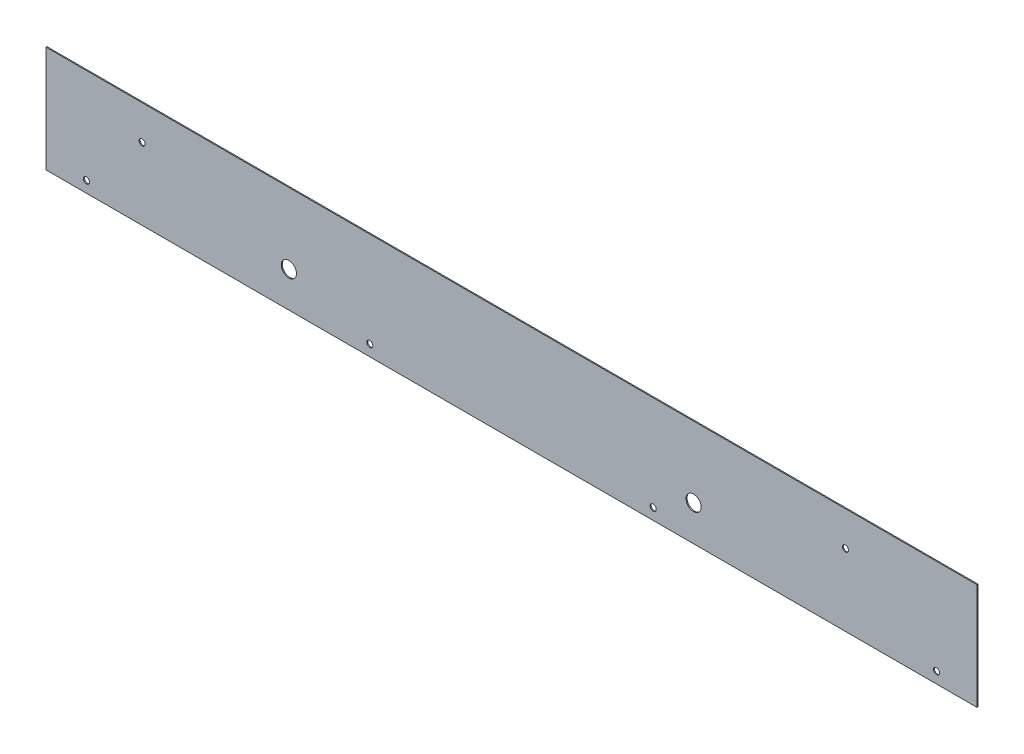
from build123d import *

# Parameters (mm, degrees)
SKETCH1_W                = 920
SKETCH1_H                = 1
EXTRUDE1_DEPTH           = 52.5
SKETCH2_R                = 7.5
CUT_EXTRUDE1_DEPTH       = 463.987310841
M5_CLEARANCE_HOLE1_D     = 6
M5_CLEARANCE_HOLE1_DEPTH = 7
M5_CLEARANCE_HOLE1_TIP   = 1.802581857


with BuildPart() as part:
    # Sketch1 → Extrude1 (new, symmetric)
    with BuildSketch(Plane(origin=(0, 0, 0), x_dir=(1, 0, 0), z_dir=(0, 1, 0))):
        Rectangle(SKETCH1_W, SKETCH1_H)
    extrude(amount=EXTRUDE1_DEPTH, both=True)

    # Sketch2 → Cut-Extrude1 (cut, through all)
    with BuildSketch(Plane.XY.offset(0.5)):
        with Locations((-220, -17.5)):
            Circle(SKETCH2_R)
        with Locations((180, -17.5)):
            Circle(SKETCH2_R)
    extrude(amount=-CUT_EXTRUDE1_DEPTH, mode=Mode.SUBTRACT)

    # M5 Clearance Hole1
    with Locations(Plane.XY.offset(0.5)):
        with Locations((-420, -41.5), (-140, -41.5), (140, -41.5), (-365, 18.5), (330, 18.5), (420, -41.5)):
            Hole(M5_CLEARANCE_HOLE1_D / 2, depth=M5_CLEARANCE_HOLE1_DEPTH)
            with Locations((0, 0, -(M5_CLEARANCE_HOLE1_DEPTH + M5_CLEARANCE_HOLE1_TIP / 2))):  # 118° drill point
                Cone(0, M5_CLEARANCE_HOLE1_D / 2, M5_CLEARANCE_HOLE1_TIP, mode=Mode.SUBTRACT)


solid = part.part
